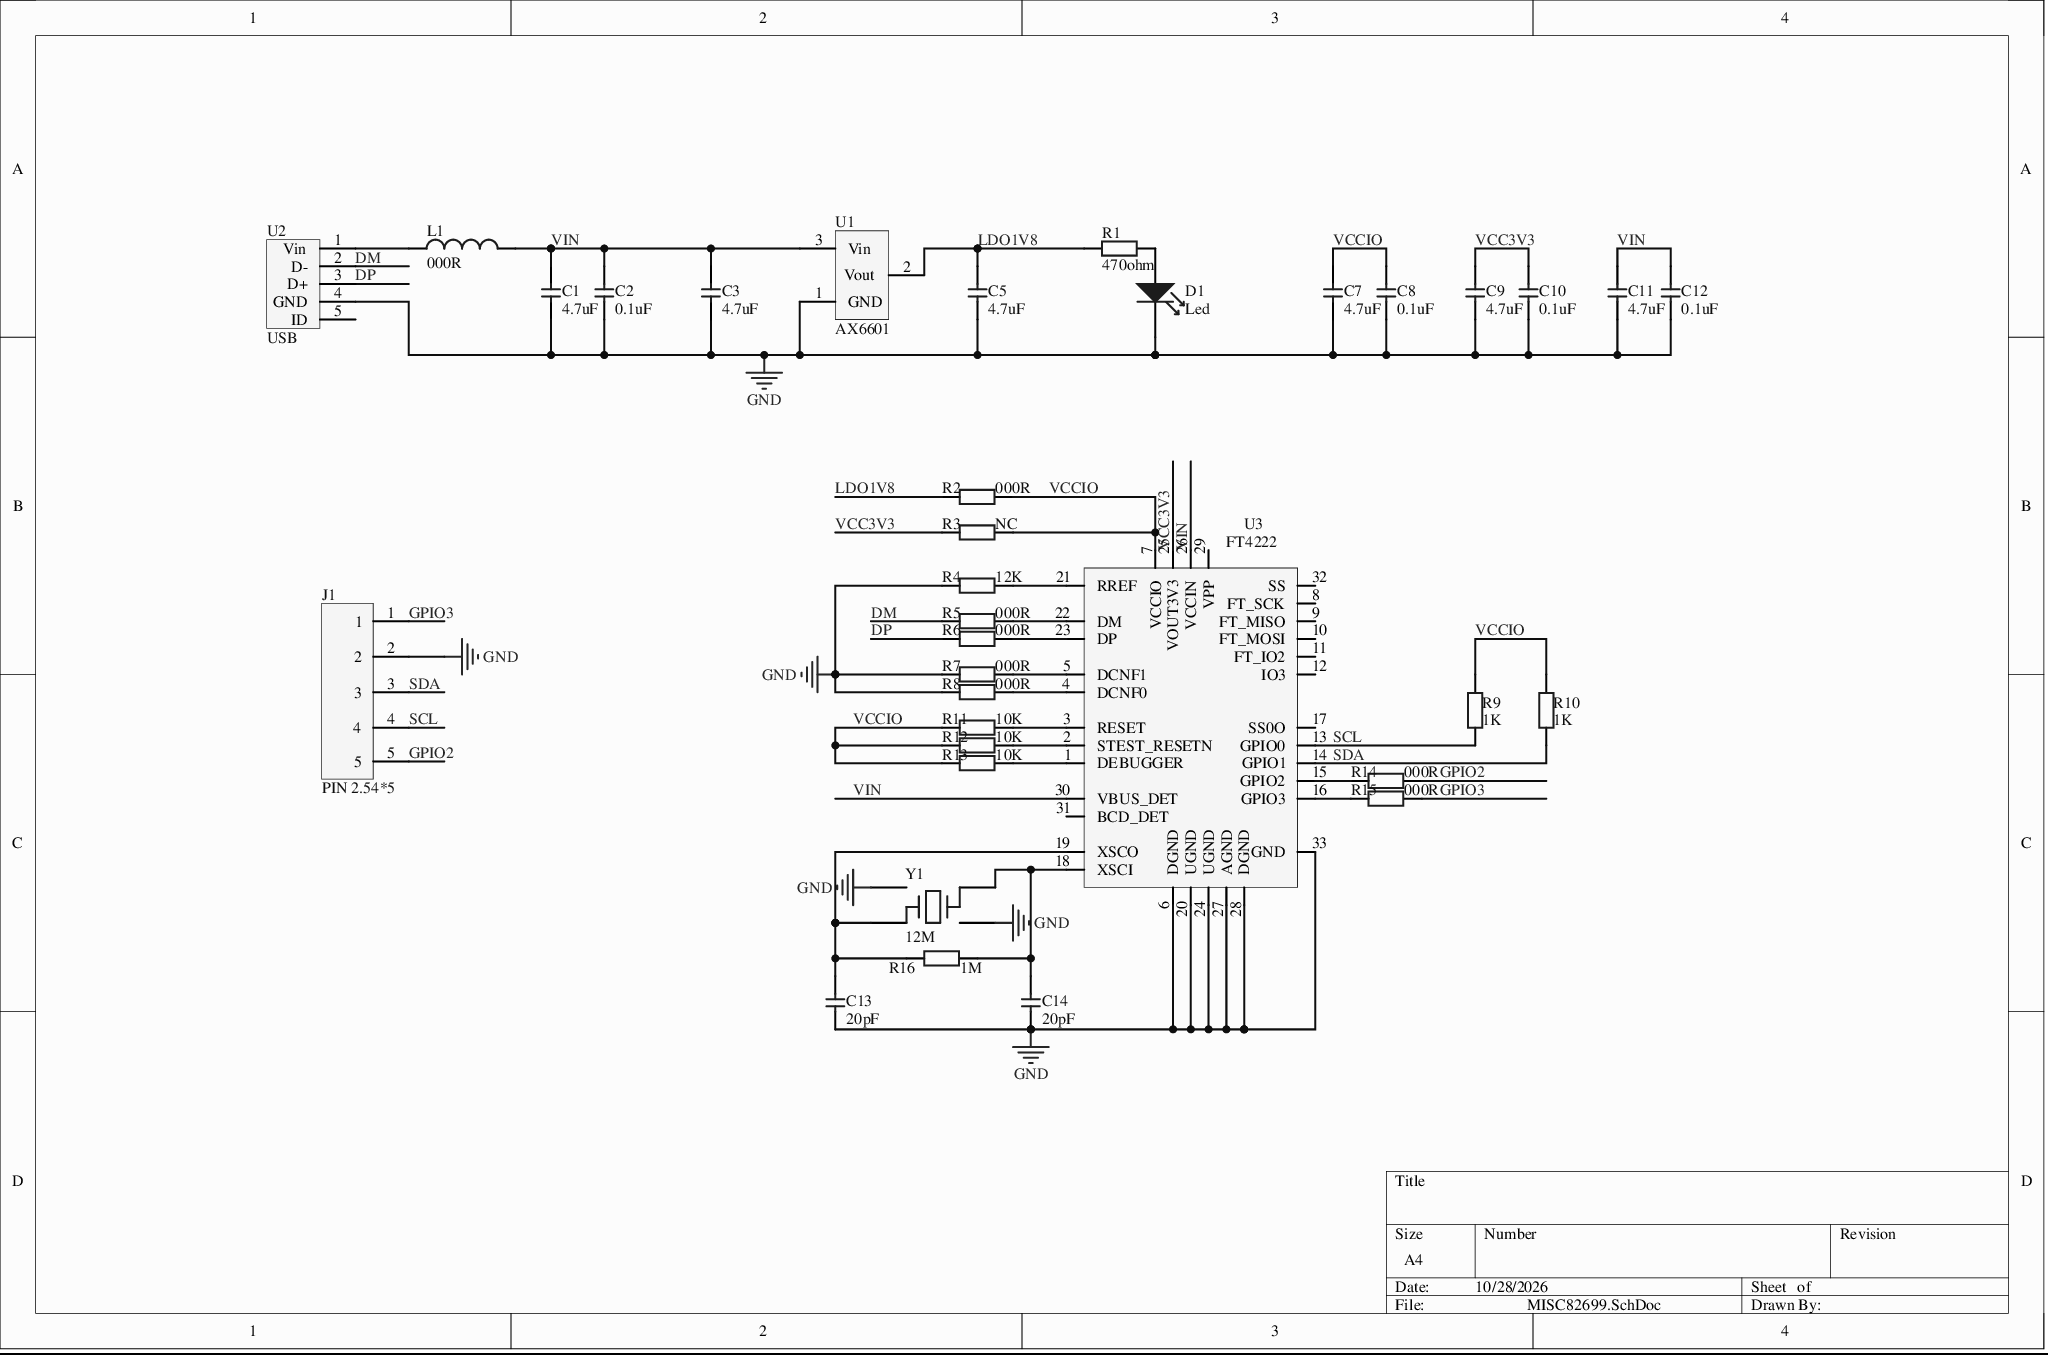
[diagram p0: MISC82699.SchDoc]
# Altium schematic sheet MISC82699.SchDoc
size A4

## Parts
C1  4.7uF  [C0402]
C2  0.1uF  [C0402]
C3  4.7uF  [C0402]
C5  4.7uF  [C0402]
C7  4.7uF  [C0402]
C8  0.1uF  [C0402]
C9  4.7uF  [C0402]
C10  0.1uF  [C0402]
C11  4.7uF  [C0402]
C12  0.1uF  [C0402]
C13  20pF  [C0402]
C14  20pF  [C0402]
D1  Led  [R0603]
J1  PIN 2.54*5  [DIP2.54*5]
L1  000R  [R0603]
R1  470ohm  [R0402]
R2  000R  [R0402]
R3  NC  [R0402]
R4  12K  [R0402]
R5  000R  [R0402]
R6  000R  [R0402]
R7  000R  [R0402]
R8  000R  [R0402]
R9  1K  [R0402]
R10  1K  [R0402]
R11  10K  [R0402]
R12  10K  [R0402]
R13  10K  [R0402]
R14  000R  [R0402]
R15  000R  [R0402]
R16  1M  [R0402]
U1  AX6601  [SOT_23]
U2  USB  [MicroUSB]
U3  FT4222  [QFN32]
Y1  12M  [XTAL_3225]

## Nets
GND: C1.1 C2.1 C3.1 C5.1 C7.1 C8.1 C9.1 C10.1 C11.1 C12.1 C13.1 C14.1 D1.1(K) J1.2 R4.1 R7.1 R8.1 U1.1(GND) U2.4(GND) U3.6(DGND) U3.20(UGND) U3.24(UGND) U3.27(AGND) U3.28(DGND) U3.33(GND) Y1.2 Y1.4
DM: R5.1 U2.2(D-)
DP: R6.1 U2.3(D+)
GPIO2: J1.5 R14.2
GPIO3: J1.1 R15.2
LDO1V8: C5.2 R1.1 R2.1 U1.2(Vout)
SCL: J1.4 R9.1 U3.13(GPIO0)
SDA: J1.3 R10.1 U3.14(GPIO1)
VCC3V3: C9.2 C10.2 R3.1 U3.25(VOUT3V3)
VCCIO: C7.2 C8.2 R2.2 R3.2 R9.2 R10.2 R11.1 R12.1 R13.1 U3.7(VCCIO)
VIN: C1.2 C2.2 C3.2 C11.2 C12.2 L1.1 U1.3(Vin) U3.26(VCCIN) U3.30(VBUS_DET)
NetC13_2: C13.2 R16.1 U3.19(XSCO) Y1.1
NetC14_2: C14.2 R16.2 U3.18(XSCI) Y1.3
NetD1_2: D1.2(A) R1.2
NetL1_2: L1.2 U2.1(Vin)
NetR4_2: R4.2 U3.21(RREF)
NetR5_2: R5.2 U3.22(DM)
NetR6_2: R6.2 U3.23(DP)
NetR7_2: R7.2 U3.5(DCNF1)
NetR8_2: R8.2 U3.4(DCNF0)
NetR11_2: R11.2 U3.3(~{RESET})
NetR12_2: R12.2 U3.2(STEST_RESETN)
NetR13_2: R13.2 U3.1(DEBUGGER)
NetR14_1: R14.1 U3.15(GPIO2)
NetR15_1: R15.1 U3.16(GPIO3)

Not connected (* = marked no-connect by the designer): U2 5(ID); U3 8(FT_SCK) 9(FT_MISO) 10(FT_MOSI) 11(FT_IO2) 12(IO3) 17(SS0O) 29(VPP) 31(BCD_DET) 32(SS)

## Library data of the parts
C1-C3 C5 C7-C14 = Cap
J1 = PIN_5
L1 = Inductor
R1-R16 = Res
U1 = LDO
U2 = Micro USB
Y1 = Crystal